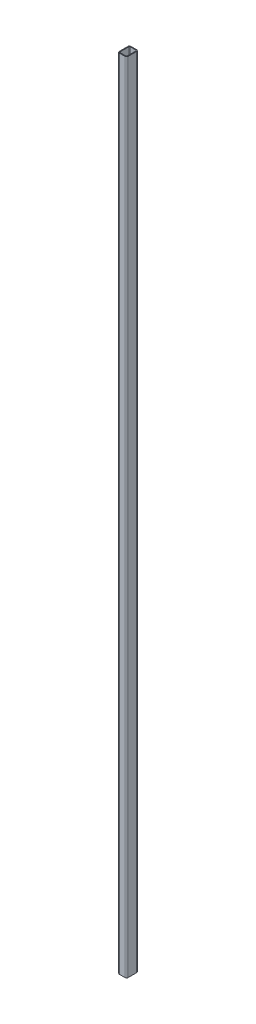
SolidWorks part; units mm, degrees
material "Q235B"
ref_plane "Front Plane" through (0, 0, 0) normal (0, 0, 1) x (1, 0, 0)
ref_plane "Top Plane" through (0, 0, 0) normal (0, 1, 0) x (1, 0, 0)
ref_plane "Right Plane" through (0, 0, 0) normal (1, 0, 0) x (0, 0, -1)
sketch "feature 17 (ProfileFeature) (+16 more in 12 files) Sketch1" plane through (0, 0, 0) normal (0, 0, 1) x (1, 0, 0)
  line L0 (0, 0) -> (0, 5500)
  dimension "D1" = 5500
other "Cold-formed Hollow Structural Rectangular Steel(gb t6728-2002) 80×60×5(1)"
ref_plane "Plane1" through (0, 0, 0) normal (0, 1, 0) x (-1, 0, 0)
sketch "Sketch1" plane through (0, 0, 0) normal (0, 1, 0) x (-1, 0, 0)
  line L0 (-20, -35) -> (20, -35)
  line L1 (-25, -30) -> (-25, 30)
  line L2 (20, 35) -> (-20, 35)
  line L3 (25, 30) -> (25, -30)
  line L4 (-20, -40) -> (20, -40)
  line L5 (-30, -30) -> (-30, 30)
  line L6 (20, 40) -> (-20, 40)
  line L7 (30, 30) -> (30, -30)
  arc A0 (30, 30) -> (20, 40) centre (20, 30) ccw
  arc A1 (20, -40) -> (30, -30) centre (20, -30) ccw
  arc A2 (-30, -30) -> (-20, -40) centre (-20, -30) ccw
  arc A3 (-20, 40) -> (-30, 30) centre (-20, 30) ccw
  arc A4 (-20, 35) -> (-25, 30) centre (-20, 30) ccw
  arc A5 (25, 30) -> (20, 35) centre (20, 30) ccw
  arc A6 (20, -35) -> (25, -30) centre (20, -30) ccw
  arc A7 (-25, -30) -> (-20, -35) centre (-20, -30) ccw
  point P0 (0, 40)
  point P1 (30, 0)
  point P2 (0, -40)
  point P3 (-30, 0)
  point P4 (-30, 40)
  point P5 (30, 40)
  point P6 (30, -40)
  point P7 (-30, -40)
  point P8 (0, 0)
  point P33 (0, 0)
  dimension "D1" = 80
  dimension "D2" = 60
  dimension "D3" = 5
  dimension "D4" = 10
